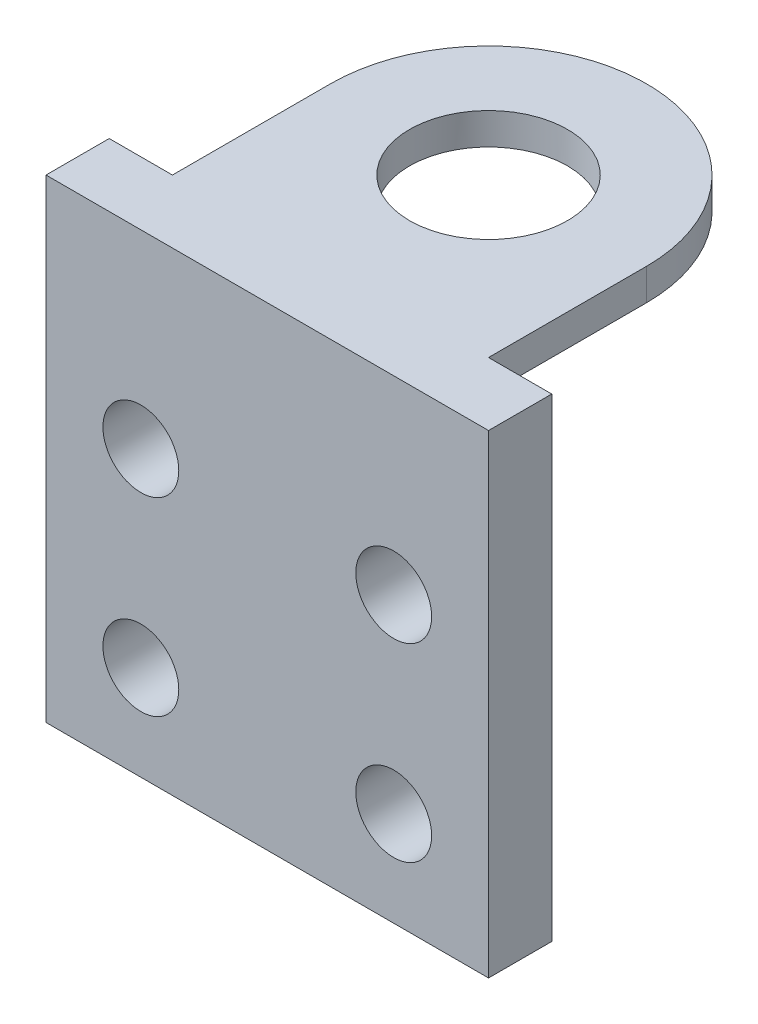
SolidWorks part; units mm, degrees
ref_plane "前视基准面" through (0, 0, 0) normal (0, 0, 1) x (1, 0, 0)
ref_plane "上视基准面" through (0, 0, 0) normal (0, 1, 0) x (1, 0, 0)
ref_plane "右视基准面" through (0, 0, 0) normal (1, 0, 0) x (0, 0, -1)
sketch "草图1" plane through (0, 0, 0) normal (0, 0, 1) x (1, 0, 0)
  line L1 (-15, 55) -> (55, 55)
  line L2 (-15, 55) -> (-15, -15)
  line L3 (-15, -15) -> (55, -15)
  line L4 (55, 55) -> (55, -15)
  circle A0 centre (0, 0) radius 6
  circle A1 centre (0, 30) radius 6
  circle A2 centre (40, 30) radius 6
  circle A3 centre (40, 0) radius 6
  dimension "D1" = 30
  dimension "D2" = 30
  dimension "D3" = 12
  dimension "D4" = 40
  dimension "D7" = 15
  dimension "D9" = 15
  dimension "D11" = 25
  dimension "D5" = 15
  dimension "D8" = 15
  dimension "D10" = 15
extrude "凸台-拉伸1" add sketch "草图1" along normal blind 10
sketch "草图2" plane through (0, 0, 10) normal (0, 0, 1) x (1, 0, 0)
  line L1 (-15, 55) -> (55, 55)
  line L2 (-15, 55) -> (-15, 60)
  line L3 (-15, 60) -> (55, 60)
  line L4 (55, 55) -> (55, 60)
extrude "凸台-拉伸2" add sketch "草图2" against normal blind 60
sketch "草图4" plane through (0, 60, 0) normal (0, 1, 0) x (1, 0, 0)
  line L0 (55, 50) -> (-15, 50) construction
  line L1 (-5, 25) -> (-5, 0)
  line L2 (45, 25) -> (45, 0)
  line L3 (45, 0) -> (55, 0)
  line L4 (55, 0) -> (55, 53.7057)
  line L5 (55, 53.7057) -> (-23.268, 53.7057)
  line L6 (-23.268, 53.7057) -> (-23.268, 0)
  line L7 (-23.268, 0) -> (-5, 0)
  line L8 (-15, 50) -> (-15, -10) construction
  circle A0 centre (20, 25) radius 12.5
  arc A1 (45, 25) -> (-5, 25) centre (20, 25) ccw
  dimension "D1" = 25
  dimension "D2" = 10
  dimension "D3" = 10
extrude "切除-拉伸1" cut sketch "草图4" against normal blind 10
